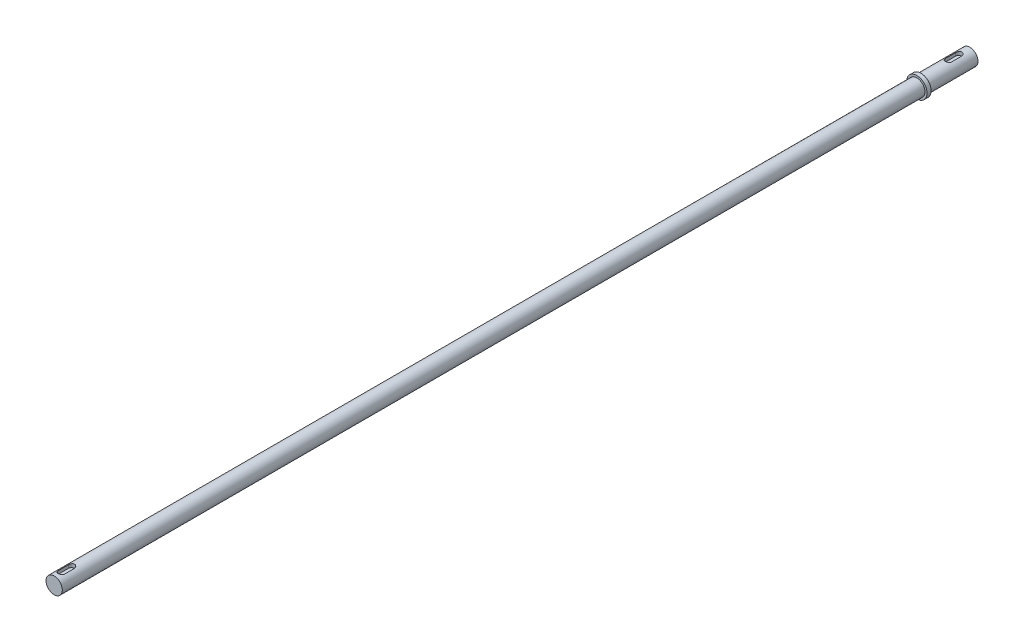
SolidWorks part; units mm, degrees
ref_plane "Front Plane" through (0, 0, 0) normal (0, 0, 1) x (1, 0, 0)
ref_plane "Top Plane" through (0, 0, 0) normal (0, 1, 0) x (1, 0, 0)
ref_plane "Right Plane" through (0, 0, 0) normal (1, 0, 0) x (0, 0, -1)
other "Configuration Table"
sketch "Sketch3" plane through (0, 0, 0) normal (0, 0, 1) x (1, 0, 0)
  circle A0 centre (0, 0) radius 4
  dimension "D1" = 8
extrude "Boss-Extrude2" add sketch "Sketch3" along normal blind 14
sketch "Sketch4" plane through (0, 0, 14) normal (0, 0, 1) x (1, 0, 0)
  circle A0 centre (0, 0) radius 4
  dimension "D1" = 8
extrude "Boss-Extrude3" add sketch "Sketch4" along normal blind 10
sketch "Sketch5" plane through (0, 0, 24) normal (0, 0, 1) x (1, 0, 0)
  circle A0 centre (0, 0) radius 5
  dimension "D1" = 10
extrude "Boss-Extrude4" add sketch "Sketch5" along normal blind 2
ref_plane "Plane1" through (0, 4, 0) normal (0, 1, 0) x (1, 0, 0)
sketch "Sketch6" plane through (0, 4, 0) normal (0, 1, 0) x (1, 0, 0)
  line L0 (0, 2.1062) -> (0, -10.5722) construction
  line L1 (0, -5.5) -> (0, -10.5) construction
  line L2 (1.5, -5.5) -> (1.5, -10.5)
  line L3 (-1.5, -5.5) -> (-1.5, -10.5)
  line L4 (4, 0) -> (-4, 0) construction
  arc A0 (1.5, -5.5) -> (-1.5, -5.5) centre (0, -5.5) ccw
  arc A1 (-1.5, -10.5) -> (1.5, -10.5) centre (0, -10.5) ccw
  point P5 (0, -8)
  dimension "D2" = 1.5
  dimension "D1" = 5
  dimension "D3" = 5.5
extrude "Cut-Extrude1" cut sketch "Sketch6" against normal blind 1.8
sketch "Sketch7" plane through (0, 0, 26) normal (0, 0, 1) x (1, 0, 0)
  circle A0 centre (0, 0) radius 4
  dimension "D1" = 8
extrude "Boss-Extrude5" add sketch "Sketch7" along normal blind 42
sketch "Sketch8" plane through (0, 0, 68) normal (0, 0, 1) x (1, 0, 0)
  circle A0 centre (0, 0) radius 4
extrude "Boss-Extrude7" add sketch "Sketch8" along normal blind 150
sketch "Sketch9" plane through (0, 0, 218) normal (0, 0, 1) x (1, 0, 0)
  circle A0 centre (0, 0) radius 4
extrude "Boss-Extrude8" add sketch "Sketch9" along normal blind 198
sketch "Sketch10" plane through (0, 0, 416) normal (0, 0, 1) x (1, 0, 0)
  circle A0 centre (0, 0) radius 4
extrude "Boss-Extrude9" add sketch "Sketch10" along normal blind 33.1
sketch "Sketch13" plane through (0, 4, 0) normal (0, 1, 0) x (1, 0, 0)
  line L0 (0, -440.6) -> (0, -445.6) construction
  line L1 (1.5, -440.6) -> (1.5, -445.6)
  line L2 (-1.5, -440.6) -> (-1.5, -445.6)
  line L3 (-4, -449.1) -> (4, -449.1) construction
  line L4 (-4, -449.1) -> (4, -449.1) construction
  arc A0 (1.5, -440.6) -> (-1.5, -440.6) centre (0, -440.6) ccw
  arc A1 (-1.5, -445.6) -> (1.5, -445.6) centre (0, -445.6) ccw
  point P3 (0, -443.1)
  dimension "D2" = 1.5
  dimension "D1" = 5
  dimension "D3" = 3.5
extrude "Cut-Extrude2" cut sketch "Sketch13" against normal blind 1.8
